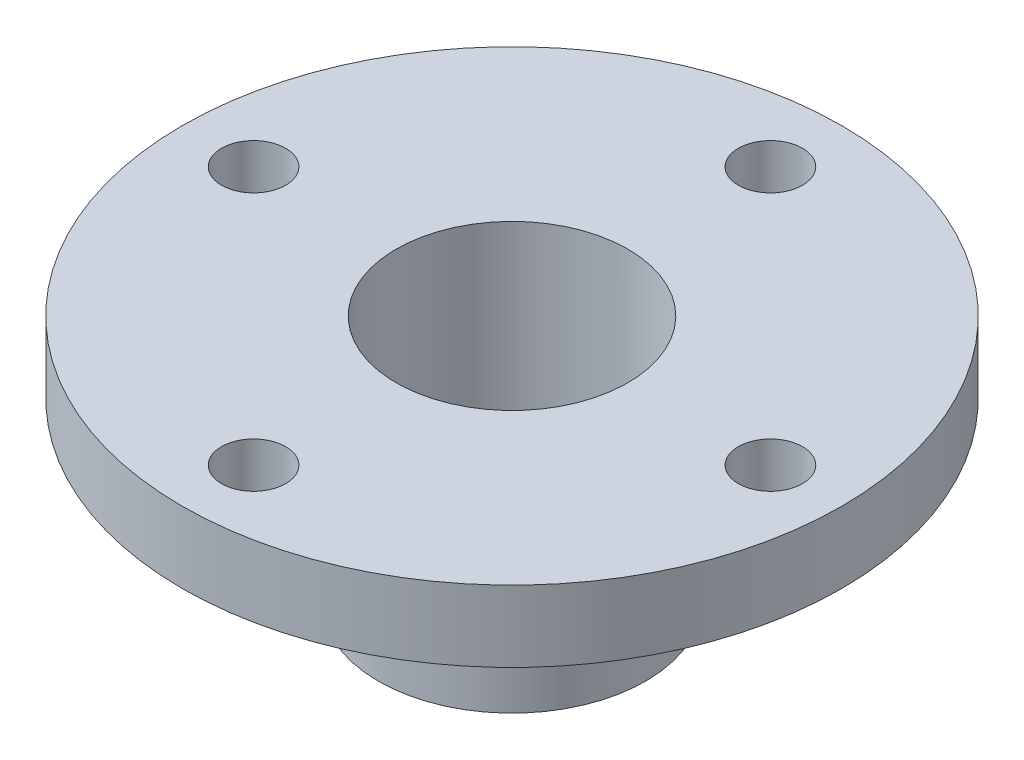
from build123d import *

# Parameters (mm, degrees)
SKETCH_1_R          = 37.5
SKETCH_1_R_2        = 32.5
EXTRUDE_1_DEPTH     = 50
SKETCH_2_R          = 92.5
SKETCH_2_R_2        = 37.5
SKETCH_2_R_3        = 9
EXTRUDE_2_DEPTH     = 20
SKETCH_3_R          = 37.5
EXTRUDE_3_DEPTH     = 20
SKETCH_4_R          = 32.5
CUT_EXTRUDE_1_DEPTH = 141.044635742


with BuildPart() as part:
    # 草图1 → 凸台-拉伸1 (new body)
    with BuildSketch(Plane(origin=(0, 0, 0), x_dir=(1, 0, 0), z_dir=(0, 1, 0))):
        with Locations(Location((0, 0, 0), (0, 0, 270))):
            Circle(SKETCH_1_R)
        with Locations(Location((0, 0, 0), (0, 0, 270))):
            Circle(SKETCH_1_R_2, mode=Mode.SUBTRACT)
    extrude(amount=EXTRUDE_1_DEPTH)



with BuildPart() as body_2:
    # 草图2 → 凸台-拉伸2 (new body)
    with BuildSketch(Plane(origin=(0, 50, 0), x_dir=(1, 0, 0), z_dir=(0, 1, 0))):
        with Locations(Location((0, 0, 0), (0, 0, 270))):
            Circle(SKETCH_2_R)
        with Locations(Location((0, 0, 0), (0, 0, 270))):
            Circle(SKETCH_2_R_2, mode=Mode.SUBTRACT)
        with Locations(Location((-72.5, 0, 0), (0, 0, 270))):
            Circle(SKETCH_2_R_3, mode=Mode.SUBTRACT)
        with Locations(Location((0, 72.5, 0), (0, 0, 270))):
            Circle(SKETCH_2_R_3, mode=Mode.SUBTRACT)
        with Locations(Location((72.5, 0, 0), (0, 0, 270))):
            Circle(SKETCH_2_R_3, mode=Mode.SUBTRACT)
        with Locations(Location((0, -72.5, 0), (0, 0, 270))):
            Circle(SKETCH_2_R_3, mode=Mode.SUBTRACT)
    extrude(amount=EXTRUDE_2_DEPTH)


with BuildPart() as part_1:
    add(part.part)

    add(body_2.part)  # 凸台-拉伸3 merges body 2
    # 草图3 → 凸台-拉伸3 (add)
    with BuildSketch(Plane(origin=(0, 50, 0), x_dir=(1, 0, 0), z_dir=(0, 1, 0))):
        with Locations(Location((0, 0, 0), (0, 0, 270))):
            Circle(SKETCH_3_R)
    extrude(amount=EXTRUDE_3_DEPTH)

    # 草图4 → 切除-拉伸1 (cut, through all)
    with BuildSketch(Plane.XZ.offset(-50)):
        with Locations(Location((0, 0, 0), (0, 0, 270))):
            Circle(SKETCH_4_R)
    extrude(amount=-CUT_EXTRUDE_1_DEPTH, mode=Mode.SUBTRACT)


solid = part_1.part
